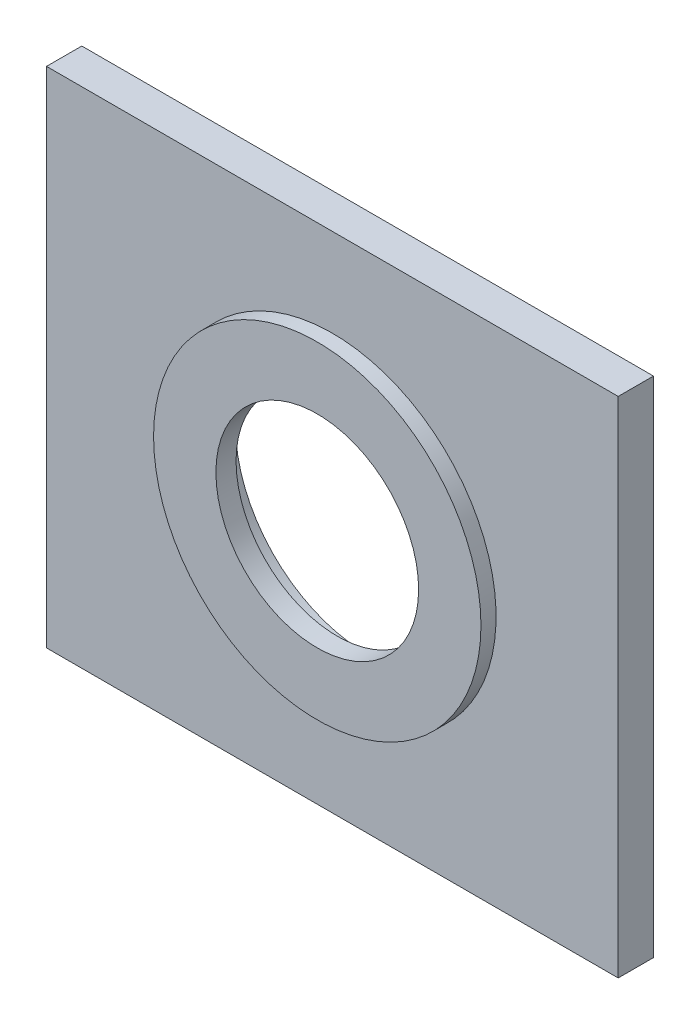
from build123d import *

# Parameters (mm, degrees)
SKETCH1_W           = 227
SKETCH1_H           = 200
BOSS_EXTRUDE1_DEPTH = 14
SKETCH2_R           = 65
BOSS_EXTRUDE2_DEPTH = 6
SKETCH3_R           = 75
SKETCH3_R_2         = 70
BOSS_EXTRUDE3_DEPTH = 8
SKETCH4_R           = 40.25
CUT_EXTRUDE1_DEPTH  = 304.830544877
SKETCH5_R           = 52.5
CUT_EXTRUDE2_DEPTH  = 12


with BuildPart() as part:
    # Sketch1 → Boss-Extrude1 (new body)
    with BuildSketch(Plane.XY):
        with Locations((113.5, 100)):
            Rectangle(SKETCH1_W, SKETCH1_H)
    extrude(amount=BOSS_EXTRUDE1_DEPTH)

    # Sketch2 → Boss-Extrude2 (add)
    with BuildSketch(Plane.XY.offset(14)):
        with Locations(Location((113.5, 100, 0), (0, 0, 180))):
            Circle(SKETCH2_R)
    extrude(amount=BOSS_EXTRUDE2_DEPTH)

    # Sketch3 → Boss-Extrude3 (add)
    with BuildSketch(Plane(origin=(0, 0, 0), x_dir=(-1, 0, 0), z_dir=(0, 0, -1))):
        with Locations((-113.5, 100)):
            Circle(SKETCH3_R)
        with Locations((-113.5, 100)):
            Circle(SKETCH3_R_2, mode=Mode.SUBTRACT)
    extrude(amount=BOSS_EXTRUDE3_DEPTH)

    # Sketch4 → Cut-Extrude1 (cut, through all)
    with BuildSketch(Plane.XY.offset(20)):
        with Locations((113.5, 100)):
            Circle(SKETCH4_R)
    extrude(amount=-CUT_EXTRUDE1_DEPTH, mode=Mode.SUBTRACT)

    # Sketch5 → Cut-Extrude2 (cut)
    with BuildSketch(Plane(origin=(0, 0, 0), x_dir=(-1, 0, 0), z_dir=(0, 0, -1))):
        with Locations((-113.5, 100)):
            Circle(SKETCH5_R)
    extrude(amount=-CUT_EXTRUDE2_DEPTH, mode=Mode.SUBTRACT)


solid = part.part
